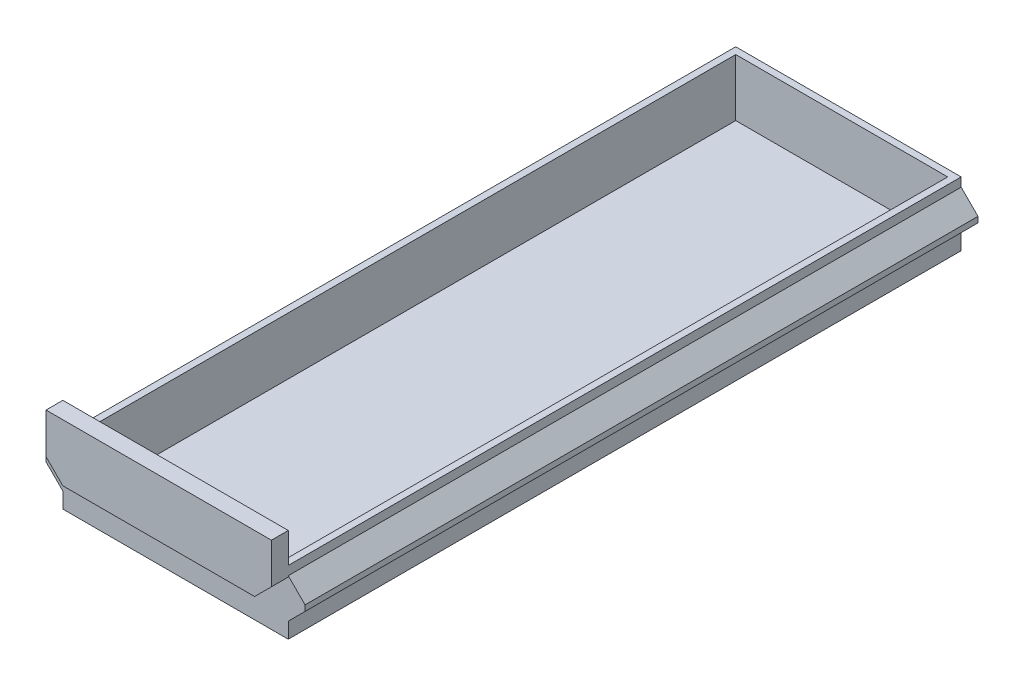
from build123d import *

# Parameters (mm, degrees)
BOSS_EXTRUDE1_DEPTH = 200
SKETCH2_W           = 63
SKETCH2_H           = 196
CUT_EXTRUDE1_DEPTH  = 17
SKETCH3_W           = 67
SKETCH3_H           = 17
BOSS_EXTRUDE2_DEPTH = 5
CHAMFER1_SIZE       = 5


with BuildPart() as part:
    # Sketch1 → Boss-Extrude1 (new body)
    with BuildSketch(Plane.XY):
        Polygon((-73, 28), (-6, 28), (-6, 32.656854249), (-1, 37.656854249), (-1, 39.353196257), (-6, 44.353196257), (-6, 47), (-73, 47), (-73, 44.353196257), (-78, 39.353196257), (-78, 37.656854249), (-73, 32.656854249), align=None)
    extrude(amount=-BOSS_EXTRUDE1_DEPTH)

    # Sketch2 → Cut-Extrude1 (cut)
    with BuildSketch(Plane(origin=(0, 47, 0), x_dir=(1, 0, 0), z_dir=(0, 1, 0))):
        with Locations((-39.5, 100)):
            Rectangle(SKETCH2_W, SKETCH2_H)
    extrude(amount=-CUT_EXTRUDE1_DEPTH, mode=Mode.SUBTRACT)

    # Sketch3 → Boss-Extrude2 (add)
    with BuildSketch(Plane.XY):
        with Locations((-39.5, 47.5)):
            Rectangle(SKETCH3_W, SKETCH3_H)
    extrude(amount=BOSS_EXTRUDE2_DEPTH)

    # Chamfer1
    chamfer1_edges = [part.edges().sort_by_distance(p)[0] for p in [
        (-73, 39, 2.5),
        (-6, 39, 2.5),
    ]]
    chamfer(chamfer1_edges, length=CHAMFER1_SIZE)


solid = part.part
